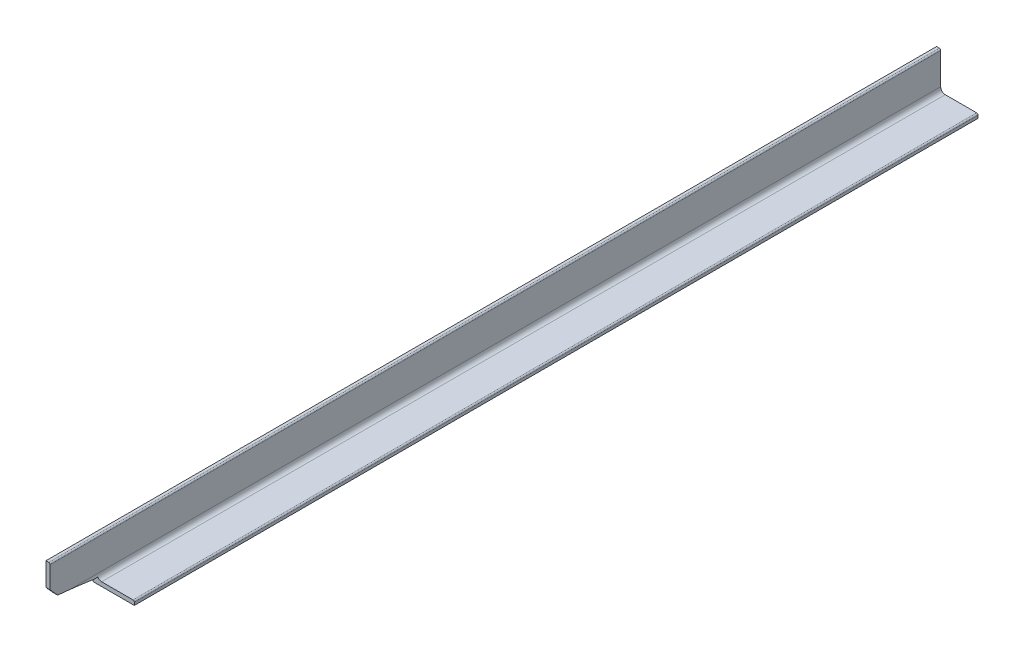
SolidWorks part; units mm, degrees
material "SPCC冷轧板喷塑"
ref_plane "前视基准面" through (0, 0, 0) normal (0, 0, 1) x (1, 0, 0)
ref_plane "上视基准面" through (0, 0, 0) normal (0, 1, 0) x (1, 0, 0)
ref_plane "右视基准面" through (0, 0, 0) normal (1, 0, 0) x (0, 0, -1)
other "Configuration Table"
sketch "草图1" plane through (0, 0, 0) normal (1, 0, 0) x (0, 0, -1)
  line L0 (0, 0) -> (1073.5, 0)
  dimension "D1" = 1073.5
other "Gbt706-2008 热轧等边角钢 050×5(1)"
ref_plane "基准面1" through (0, 0, 0) normal (0, 0, -1) x (0, 1, 0)
sketch "Sketch1" plane through (0, 0, 0) normal (0, 0, -1) x (0, 1, 0)
  line L0 (0, 0) -> (0, 50)
  line L1 (0, 25) -> (5, 25) construction
  line L2 (5, 48.3333) -> (5, 10.5)
  line L3 (10.5, 5) -> (48.3333, 5)
  line L4 (25, 5) -> (25, 0) construction
  line L5 (50, 0) -> (0, 0)
  line L6 (0, 50) -> (3.3333, 50)
  line L7 (50, 0) -> (50, 3.3333)
  arc A0 (50, 3.3333) -> (48.3333, 5) centre (48.3333, 3.3333) ccw
  arc A1 (3.3333, 50) -> (5, 48.3333) centre (3.3333, 48.3333) cw
  arc A2 (10.5, 5) -> (5, 10.5) centre (10.5, 10.5) cw
  point P10 (25, 0)
  point P14 (0, 25)
  point P15 (5, 25)
  point P16 (25, 5)
  point P17 (5, 50)
  point P18 (50, 5)
  point P21 (50, 5)
  point P24 (5, 50)
  point P25 (0, 0)
sketch "草图3" plane through (0, 0, 0) normal (-1, 0, 0) x (0, 0, 1)
  line L0 (-56.5, 0) -> (-56.5, 7.5014)
  line L1 (-1073.5, 0) -> (0, 0) construction
  line L2 (-56.5, 2.5288) -> (-56.5, 0) construction
  line L3 (-3234.9774, 7.5014) -> (-52.0226, 7.5014) construction
  line L4 (-56.5, 7.5014) -> (-52.0226, 7.5014)
  line L5 (-52.0226, 7.5014) -> (-8.9547, 12.028)
  line L6 (-8.9547, 12.028) -> (0, 21.9732)
  line L7 (0, 0) -> (0, 50) construction
  line L8 (-3287, 21.9732) -> (0, 21.9732) construction
  line L9 (0, 21.9732) -> (20, 21.9732)
  line L10 (20, 21.9732) -> (20, -8.0268)
  line L11 (20, -8.0268) -> (-56.5, -8.0268)
  line L12 (-56.5, -8.0268) -> (-56.5, 0)
  dimension "D1" = 30
  dimension "D2" = 20
extrude "切除-拉伸1" cut sketch "草图3" against normal up to next
equation "\"D2@Sketch1\"= \"D1@Sketch1\" / 3"
